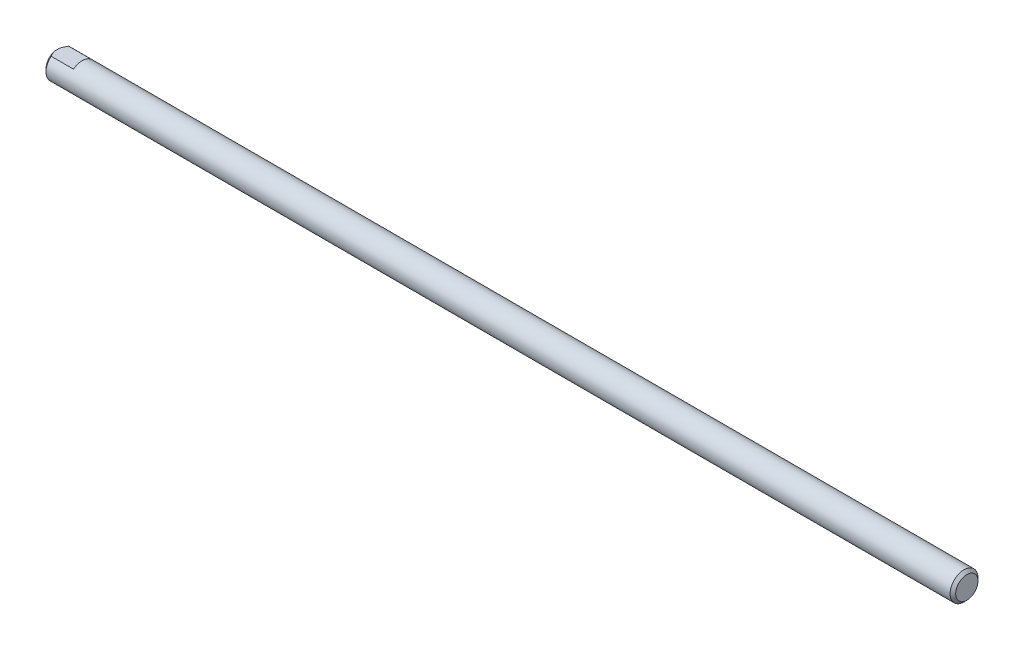
from build123d import *

# Parameters (mm, degrees)
SKETCH1_R               = 5
BOSS_EXTRUDE1_DEPTH     = 326
CHAMFER1_SIZE           = 1
CUT_EXTRUDE1_DEPTH      = 327.076678099
CUT_EXTRUDE1_DEPTH_BACK = 327.076678099
SKETCH8_W               = 156.812935598
SKETCH8_H               = 4.242810574
SKETCH8_H_2             = 7.575578147


with BuildPart() as part:
    # Sketch1 → Boss-Extrude1 (new body)
    with BuildSketch(Plane(origin=(0, 0, 0), x_dir=(0, 0, -1), z_dir=(1, 0, 0))):
        Circle(SKETCH1_R)
    extrude(amount=BOSS_EXTRUDE1_DEPTH)

    # Chamfer1
    chamfer1_edges = [part.edges().sort_by_distance(p)[0] for p in [
        (0, 0, 5),
        (326, 0, 5),
    ]]
    chamfer(chamfer1_edges, length=CHAMFER1_SIZE)

    # Sketch8 → Cut-Extrude1 (cut, two sides: drawn at the far end of the back side and taken through both)
    with BuildSketch(Plane.XY.offset(-CUT_EXTRUDE1_DEPTH_BACK)):
        with Locations((413.406467799, 6.021405287)):
            Rectangle(SKETCH8_W, SKETCH8_H)
        with Locations((413.406467799, -6.021405287)):
            Rectangle(SKETCH8_W, SKETCH8_H)
        with Locations((-69.406467799, 7.687789074)):
            Rectangle(SKETCH8_W, SKETCH8_H_2)
        with Locations((-69.406467799, -7.687789074)):
            Rectangle(SKETCH8_W, SKETCH8_H_2)
    extrude(amount=CUT_EXTRUDE1_DEPTH + CUT_EXTRUDE1_DEPTH_BACK, mode=Mode.SUBTRACT)


solid = part.part
